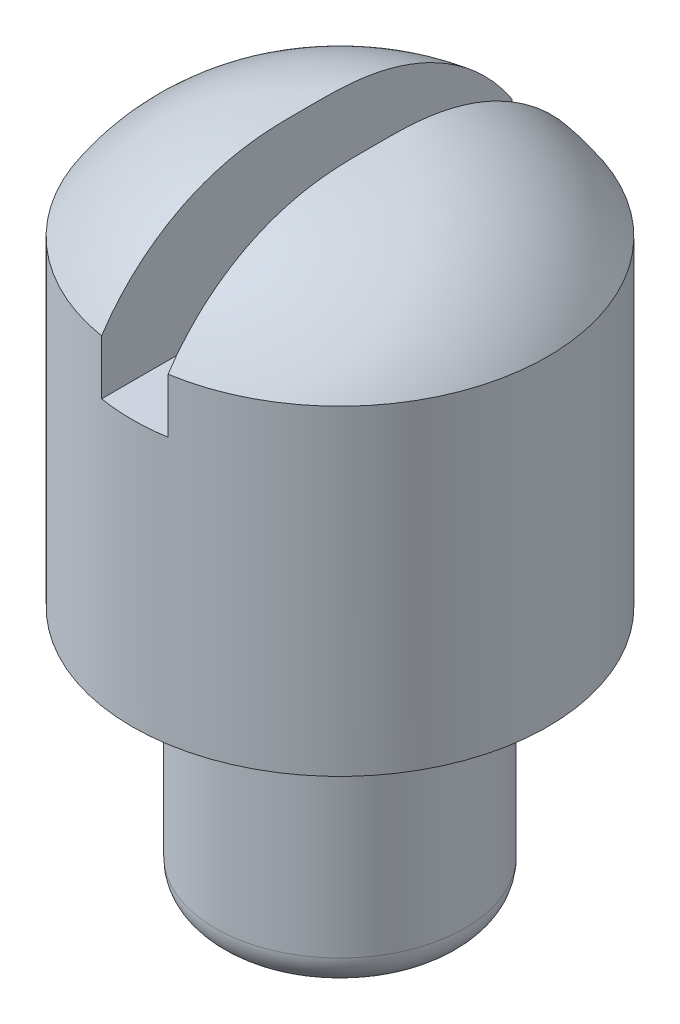
from build123d import *

# Parameters (mm, degrees)
FILLET1_R          = 0.4
FILLET2_R          = 0.4
SKETCH3_W          = 0.8
SKETCH3_H          = 1.8
CUT_EXTRUDE1_DEPTH = 5


with BuildPart() as part:
    # Sketch1 → Revolve1 (revolve)
    with BuildSketch(Plane.XY, mode=Mode.PRIVATE) as revolve1_sk:
        with BuildLine():
            Line((0, 0), (-1.5, 0))
            Line((-1.5, 0), (-1.5, 3))
            Line((-1.5, 3), (-2.5, 3))
            Line((-2.5, 3), (-2.5, 6.856465997))
            ThreePointArc((-2.5, 6.856465997), (-1.595582496, 7.695582496), (-0.4, 8))
            Line((-0.4, 8), (0, 8))
            Line((0, 8), (0, 5.056465997))
            Line((0, 5.056465997), (0, 0))
        make_face()
    revolve(revolve1_sk.sketch.rotate(Axis((0, 5.056465997, 0), (0, -1, 0)), 270), axis=Axis((0, 5.056465997, 0), (0, -1, 0)))

    # Fillet1
    fillet1_edges = [part.edges().sort_by_distance(p)[0] for p in [
        (0, 3, -1.5),
    ]]
    fillet(fillet1_edges, radius=FILLET1_R)

    # Fillet2
    fillet2_edges = [part.edges().sort_by_distance(p)[0] for p in [
        (0, 0, -1.5),
    ]]
    fillet(fillet2_edges, radius=FILLET2_R)

    # Sketch3 → Cut-Extrude1 (cut, symmetric)
    with BuildSketch(Plane.XY):
        with Locations((0, 7.1)):
            Rectangle(SKETCH3_W, SKETCH3_H)
    extrude(amount=CUT_EXTRUDE1_DEPTH, both=True, mode=Mode.SUBTRACT)


solid = part.part
